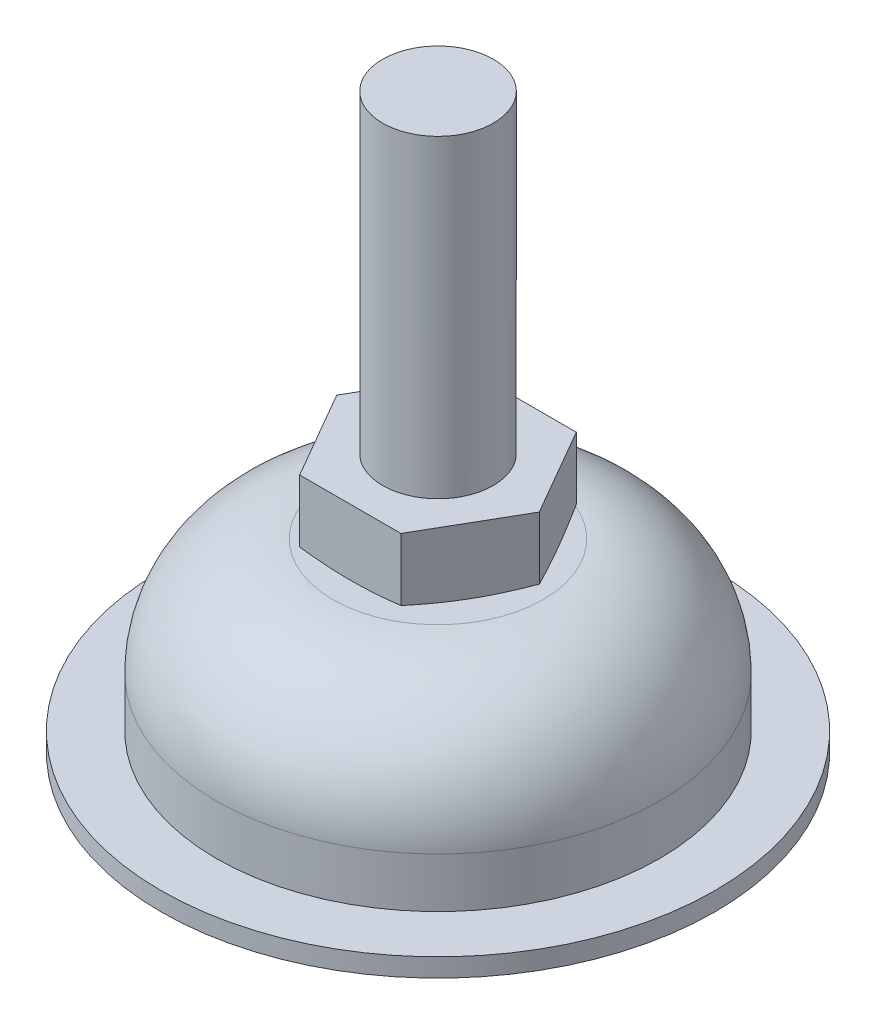
from build123d import *

# Parameters (mm, degrees)
SKETCH3_R          = 12.35
CUT_EXTRUDE1_DEPTH = 9
SKETCH5_R          = 16.85236212
CUT_EXTRUDE2_DEPTH = 66


with BuildPart() as part:
    # Sketch1 → Revolve1 (revolve)
    with BuildSketch(Plane.XY, mode=Mode.PRIVATE) as revolve1_sk:
        with BuildLine():
            Line((0, 28), (11.875, 28))
            Line((11.875, 28), (11.875, 21.461538462))
            Line((11.875, 21.461538462), (6, 20))
            Line((6, 20), (11.4, 20))
            ThreePointArc((11.4, 20), (20.309545443, 16.309545443), (24, 7.4))
            Line((24, 7.4), (24, 2))
            Line((24, 2), (30, 2))
            Line((30, 2), (30, 0))
            Line((30, 0), (0, 0))
            Line((0, 0), (0, 28))
        make_face()
    revolve(revolve1_sk.sketch.rotate(Axis((0, 0, 0), (0, 1, 0)), 180), axis=Axis((0, 0, 0), (0, 1, 0)))

    # Sketch2 → Revolve2 (revolve)
    with BuildSketch(Plane.XY, mode=Mode.PRIVATE) as revolve2_sk:
        Polygon((0, 128), (4.9265, 128), (6, 126.9265), (6, 28), (0, 28), align=None)
    revolve(revolve2_sk.sketch.rotate(Axis((0, 28, 0), (0, 1, 0)), 180), axis=Axis((0, 28, 0), (0, 1, 0)))

    # Sketch3 → Cut-Extrude1 (cut)
    with BuildSketch(Plane(origin=(0, 20, 0), x_dir=(1, 0, 0), z_dir=(0, 1, 0))):
        Circle(SKETCH3_R)
        Polygon((-10.969655115, 0), (-5.484827557, -9.5), (5.484827557, -9.5), (10.969655115, 0), (5.484827557, 9.5), (-5.484827557, 9.5), align=None, mode=Mode.SUBTRACT)
    extrude(amount=CUT_EXTRUDE1_DEPTH, mode=Mode.SUBTRACT)

    # Sketch4 → Cut-Revolve1 (revolve, cut)
    with BuildSketch(Plane.XY, mode=Mode.PRIVATE) as cut_revolve1_sk:
        with BuildLine():
            Line((0, 18), (11.4, 18))
            ThreePointArc((11.4, 18), (19.461017306, 14.661017306), (22.8, 6.6))
            Line((22.8, 6.6), (22.8, -1))
            Line((22.8, -1), (0, -1))
            Line((0, -1), (0, 18))
        make_face()
    revolve(cut_revolve1_sk.sketch.rotate(Axis((0, -1, 0), (0, 1, 0)), 270), axis=Axis((0, -1, 0), (0, 1, 0)), mode=Mode.SUBTRACT)

    # Sketch5 → Cut-Extrude2 (cut)
    with BuildSketch(Plane(origin=(0, 128, 0), x_dir=(1, 0, 0), z_dir=(0, 1, 0))):
        Circle(SKETCH5_R)
    extrude(amount=-CUT_EXTRUDE2_DEPTH, mode=Mode.SUBTRACT)


solid = part.part
